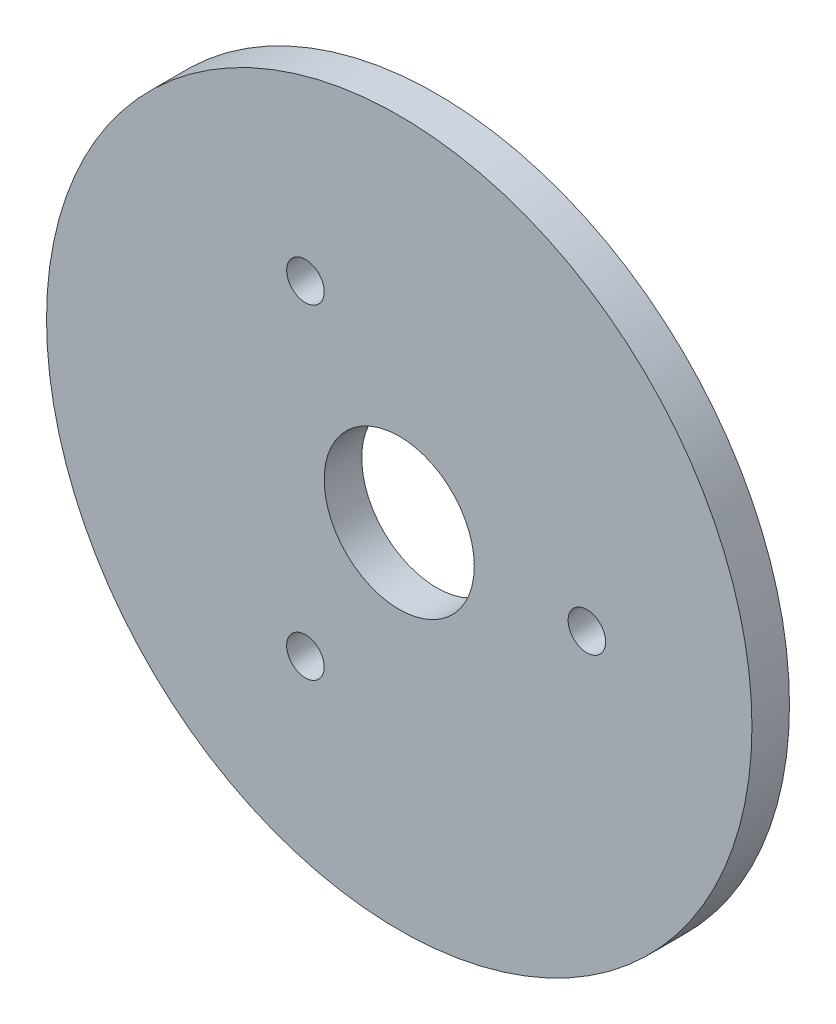
from build123d import *

# Parameters (mm, degrees)
SKETCH1_R           = 47
SKETCH1_R_2         = 10
SKETCH1_R_3         = 2.5
BOSS_EXTRUDE1_DEPTH = 5


with BuildPart() as part:
    # Sketch1 → Boss-Extrude1 (new body)
    with BuildSketch(Plane.XY):
        Circle(SKETCH1_R)
        Circle(SKETCH1_R_2, mode=Mode.SUBTRACT)
        with Locations((25, 0)):
            Circle(SKETCH1_R_3, mode=Mode.SUBTRACT)
        with Locations((-12.5, -21.650635095)):
            Circle(SKETCH1_R_3, mode=Mode.SUBTRACT)
        with Locations((-12.5, 21.650635095)):
            Circle(SKETCH1_R_3, mode=Mode.SUBTRACT)
    extrude(amount=BOSS_EXTRUDE1_DEPTH)


solid = part.part
